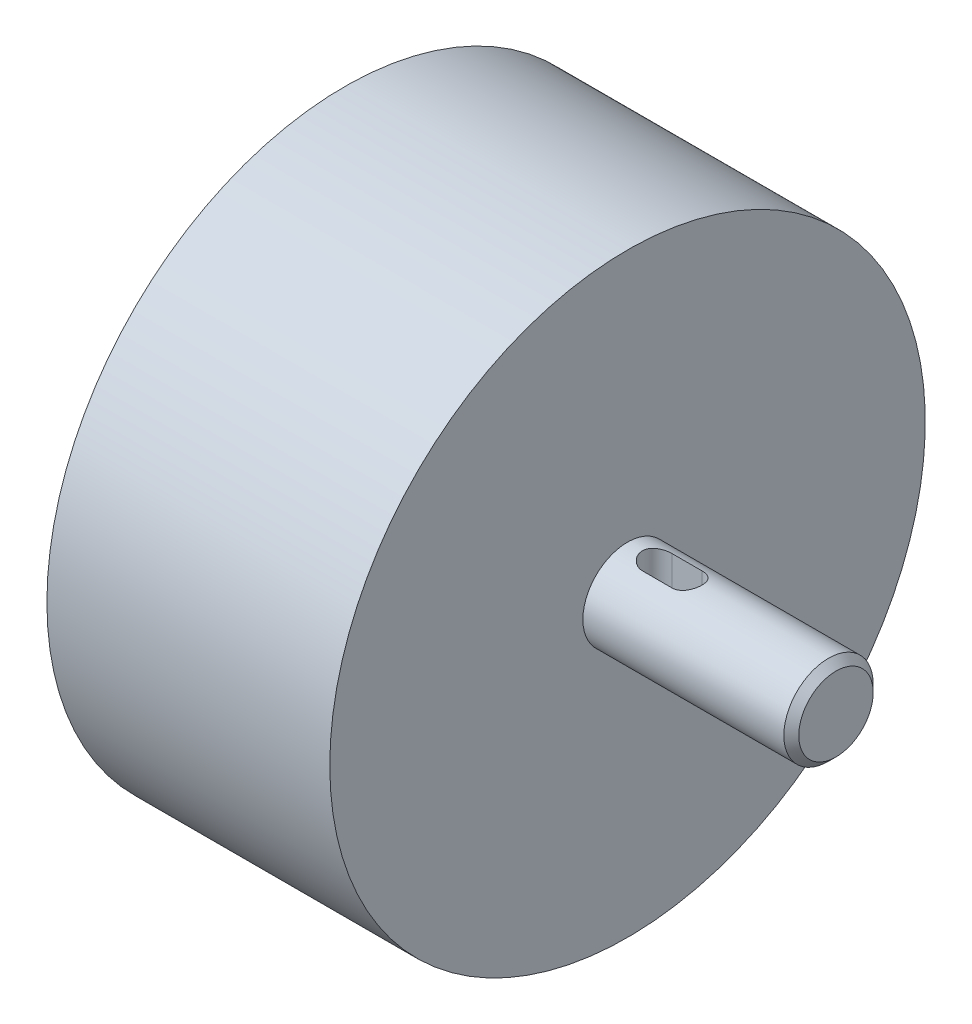
SolidWorks part; units mm, degrees
ref_plane "Front" through (0, 0, 0) normal (0, 0, 1) x (1, 0, 0)
ref_plane "Top" through (0, 0, 0) normal (0, 1, 0) x (1, 0, 0)
ref_plane "Right" through (0, 0, 0) normal (1, 0, 0) x (0, 0, -1)
sketch "Sketch1" plane through (0, 0, 0) normal (0, 1, 0) x (1, 0, 0)
  line L0 (-19, 0) -> (16.5832, 0) construction
  line L1 (0, -3) -> (14, -3)
  line L2 (-19, 0) -> (14, 0)
  line L3 (-19, 0) -> (-19, -20)
  line L4 (-19, -20) -> (0, -20)
  line L5 (0, -3) -> (0, -20)
  line L6 (14, -3) -> (14, 0)
  dimension "D1" = 40
  dimension "D2" = 19
  dimension "D3" = 14
  dimension "D4" = 6
revolve "Revolve1" add sketch "Sketch1" angle 360 about L0
sketch "Sketch2" plane through (-19, 0, 0) normal (1, 0, 0) x (0, 0, -1)
  line L1 (6.75, -6.75) -> (-6.75, -6.75)
  line L2 (6.75, -6.75) -> (6.75, 6.75)
  line L3 (6.75, 6.75) -> (-6.75, 6.75)
  line L4 (-6.75, -6.75) -> (-6.75, 6.75)
  line L5 (6.75, -6.75) -> (-6.75, 6.75) construction
  line L6 (6.75, 6.75) -> (-6.75, -6.75) construction
  point P0 (0, 0)
  dimension "D1" = 13.5
extrude "Cut-Extrude1" cut sketch "Sketch2" along normal blind 9
chamfer "Chamfer1" distance 1 angle 45 4 edges at (-19, 0, 6.75) (-19, -6.75, 0) (-19, 0, -6.75) (-19, 6.75, 0)
sketch "Sketch3" plane through (0, 0, 0) normal (0, 1, 0) x (1, 0, 0)
  line L0 (2, 0) -> (4, 0) construction
  line L1 (2, 1) -> (4, 1)
  line L2 (2, -1) -> (4, -1)
  line L3 (0, -20) -> (0, 20) construction
  arc A0 (2, 1) -> (2, -1) centre (2, 0) ccw
  arc A1 (4, -1) -> (4, 1) centre (4, 0) ccw
  point P3 (3, 0)
  dimension "D3" = 1
  dimension "D1" = 2
  dimension "D2" = 2
extrude "Cut-Extrude2" cut sketch "Sketch3" against normal through all and the other way through all
chamfer "Chamfer2" distance 0.5 angle 45 1 edges at (14, 0, 3)
